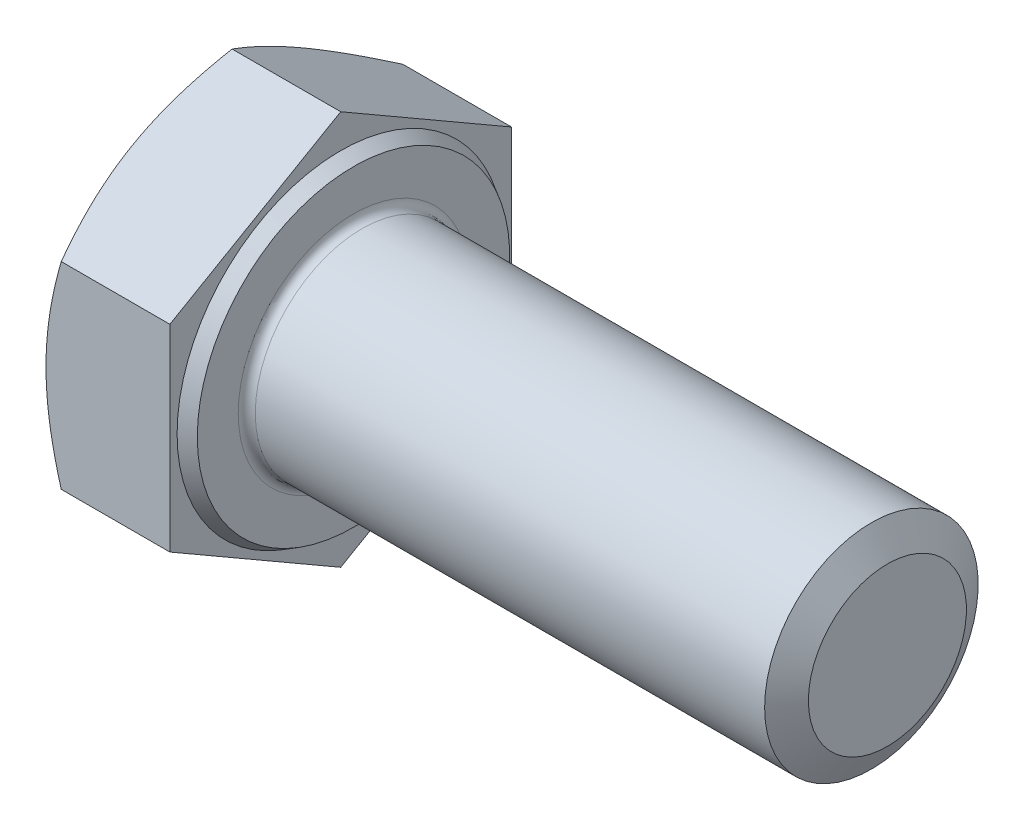
from build123d import *

# Parameters (mm, degrees)
EXTRUDE_390_DEPTH = 6.4
FILLET_1290_R     = 0.4


with BuildPart() as part:
    # 草图1 → Extrude 390 (new body)
    with BuildSketch(Plane(origin=(0, 0, 0), x_dir=(0, 0, -1), z_dir=(1, 0, 0))):
        Polygon((8, 4.618802154), (8, -4.618802154), (0, -9.237604307), (-8, -4.618802154), (-8, 4.618802154), (0, 9.237604307), align=None)
    extrude(amount=EXTRUDE_390_DEPTH)

    # 草图2 → 凸台-旋转1 (revolve)
    with BuildSketch(Plane.XY, mode=Mode.PRIVATE) as revolve_1_sk:
        Polygon((0, 0), (31.4, 0), (31.4, 3.701), (31.4, 5), (0, 5), align=None)
    revolve(revolve_1_sk.sketch.rotate(Axis((0, 0, 0), (1, 0, 0)), 90), axis=Axis((0, 0, 0), (1, 0, 0)))

    # 草图3 → 切除-旋转1 (revolve, cut)
    with BuildSketch(Plane.XY):
        Polygon((0, 8), (3.601282526, 14.237604307), (3.601282526, 19.237604307), (-10, 19.237604307), (-10, 8), align=None)
    revolve(axis=Axis((0, 0, 0), (1, 0, 0)), mode=Mode.SUBTRACT)

    # 草图4 → 切除-旋转3 (revolve, cut)
    with BuildSketch(Plane.XY, mode=Mode.PRIVATE) as cut_revolve_3_sk:
        Polygon((6.4, 7.315), (5.8, 7.661410162), (5.8, 9.237604307), (6.4, 9.237604307), align=None)
    revolve(cut_revolve_3_sk.sketch.rotate(Axis((0, 0, 0), (1, 0, 0)), 90), axis=Axis((0, 0, 0), (1, 0, 0)), mode=Mode.SUBTRACT)

    # Fillet 1290
    fillet_1290_edges = [part.edges().sort_by_distance(p)[0] for p in [
        (6.4, 0, -5),
    ]]
    fillet(fillet_1290_edges, radius=FILLET_1290_R)

    # 草图6 → 切除-旋转4 (revolve, cut)
    with BuildSketch(Plane.XY, mode=Mode.PRIVATE) as cut_revolve_4_sk:
        Polygon((30.65, 5), (32.15, 5), (31.4, 3.700961894), align=None)
    revolve(cut_revolve_4_sk.sketch.rotate(Axis((0, 0, 0), (1, 0, 0)), 90), axis=Axis((0, 0, 0), (1, 0, 0)), mode=Mode.SUBTRACT)


solid = part.part
